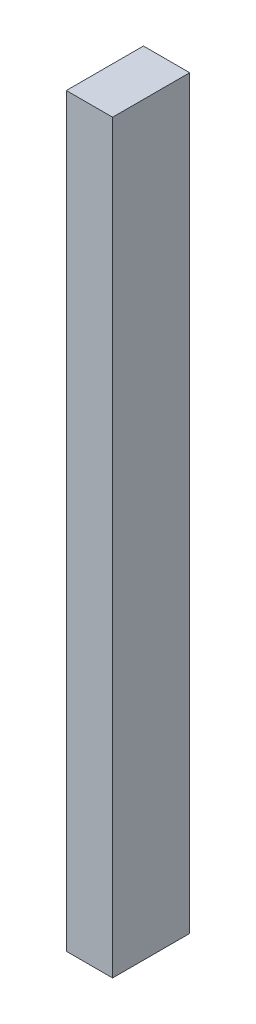
SolidWorks part; units mm, degrees
ref_plane "前视基准面" through (0, 0, 0) normal (0, 0, 1) x (1, 0, 0)
ref_plane "上视基准面" through (0, 0, 0) normal (0, 1, 0) x (1, 0, 0)
ref_plane "右视基准面" through (0, 0, 0) normal (1, 0, 0) x (0, 0, -1)
sketch "草图1" plane through (0, 0, 0) normal (0, 0, 1) x (1, 0, 0)
  line L1 (-15, 241.75) -> (15, 241.75)
  line L2 (-15, 241.75) -> (-15, -241.75)
  line L3 (-15, -241.75) -> (15, -241.75)
  line L4 (15, 241.75) -> (15, -241.75)
  line L5 (-15, 241.75) -> (15, -241.75) construction
  line L6 (-15, -241.75) -> (15, 241.75) construction
  point P0 (0, 0)
  dimension "D1" = 30
  dimension "D2" = 483.5
extrude "凸台-拉伸1" add sketch "草图1" along normal blind 50
